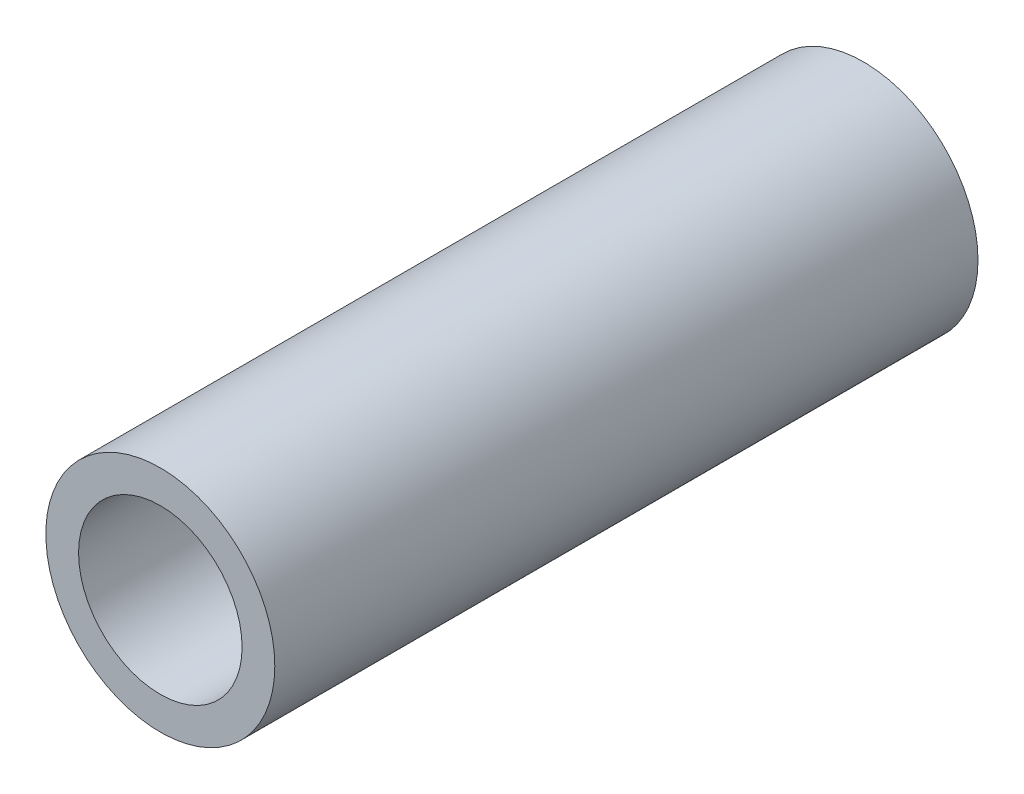
from build123d import *

# Parameters (mm, degrees)
SKETCH_1_R      = 7
SKETCH_1_R_2    = 5
EXTRUDE_1_DEPTH = 43


with BuildPart() as part:
    # 草图1 → 凸台-拉伸1 (new body)
    with BuildSketch(Plane.XY):
        Circle(SKETCH_1_R)
        Circle(SKETCH_1_R_2, mode=Mode.SUBTRACT)
    extrude(amount=EXTRUDE_1_DEPTH)


solid = part.part
